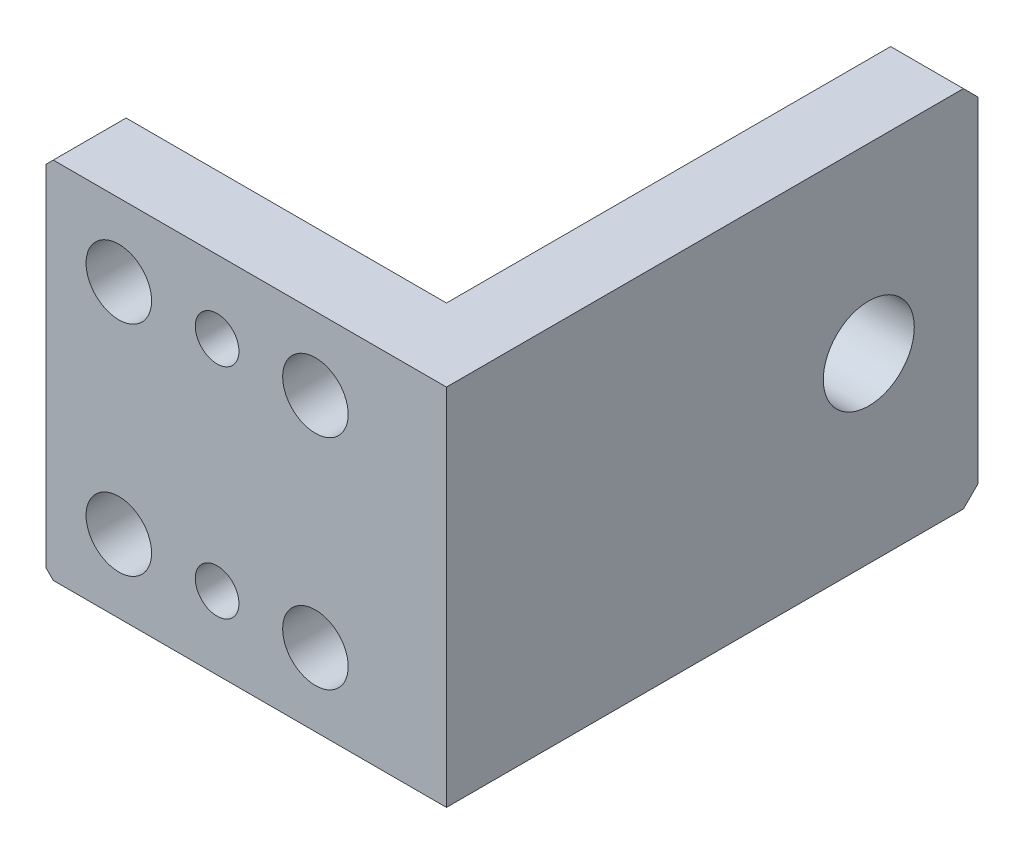
SolidWorks part; units mm, degrees
material "Q235-A"
ref_plane "Front Plane" through (0, 0, 0) normal (0, 0, 1) x (1, 0, 0)
ref_plane "Top Plane" through (0, 0, 0) normal (0, 1, 0) x (1, 0, 0)
ref_plane "Right Plane" through (0, 0, 0) normal (1, 0, 0) x (0, 0, -1)
sketch "Sketch1" plane through (0, 0, 0) normal (0, 0, 1) x (1, 0, 0)
  line L1 (-27.5, 25) -> (27.5, 25)
  line L2 (-27.5, 25) -> (-27.5, -25)
  line L3 (-27.5, -25) -> (27.5, -25)
  line L4 (27.5, 25) -> (27.5, -25)
  line L5 (-27.5, 25) -> (27.5, -25) construction
  line L6 (-27.5, -25) -> (27.5, 25) construction
  point P0 (0, 0)
  dimension "D1" = 55
  dimension "D2" = 50
extrude "Boss-Extrude1" add sketch "Sketch1" along normal blind 10
sketch "Sketch4" plane through (0, 0, 0) normal (0, 0, -1) x (-1, 0, 0)
  line L0 (-27.5, 25) -> (27.5, 25) construction
  line L1 (-17.5, 25) -> (-27.5, 25)
  line L2 (-17.5, 25) -> (-17.5, -25)
  line L3 (-17.5, -25) -> (-27.5, -25)
  line L4 (-27.5, 25) -> (-27.5, -25)
  line L5 (27.5, -25) -> (-27.5, -25) construction
  line L6 (-27.5, -25) -> (-27.5, 25) construction
  dimension "D1" = 10
extrude "Boss-Extrude2" add sketch "Sketch4" along normal blind 63
hole_wizard "M8 Clearance Hole1" positions "Sketch6" profile "Sketch7" hole size "M8" standard "GB"
sketch "Sketch6" plane through (0, 0, 0) normal (0, 0, -1) x (-1, 0, 0)
  line L0 (27.5, 0) -> (-40.8743, 0) construction
  line L1 (27.5, 25) -> (27.5, -25) construction
  line L3 (-17.5, -25) -> (-17.5, 25) construction
  point P0 (17.5, -15)
  point P2 (17.5, 15)
  point P4 (-9.5, -15)
  point P6 (-9.5, 15)
  dimension "D1" = 30
  dimension "D2" = 27
  dimension "D3" = 8
sketch "Sketch7" plane through (-17.5, -15, 0) normal (1, 0, 0) x (0, 1, 0)
  line L0 (0, 0) -> (0, 123.7039)
  line L1 (0, 123.7039) -> (4.5, 121)
  line L2 (4.5, 121) -> (4.5, 0)
  line L5 (4.5, 0) -> (0, 0)
  line L10 (0, 123.7039) -> (-4.5, 121) construction
  line L11 (0, -6.35) -> (0, 107.95) construction
  dimension "孔直径" = 9
  dimension "孔深度" = 121
  dimension "导头角度" = 118
chamfer "Chamfer1" distance 1 angle 45 2 edges at (-27.5, -25, 5) (-27.5, 25, 5)
hole_wizard "M14x1.5 Tapped Hole1" positions "Sketch9" profile "Sketch10" tap size "M14x1.5" standard "GB" end condition through all
sketch "Sketch9" plane through (27.5, 0, 0) normal (1, 0, 0) x (0, 0, -1)
  line L0 (-10, 0) -> (102.6904, 0)
  line L1 (-10, -25) -> (-10, 25) construction
  line L2 (63, 25) -> (63, -25) construction
  point P0 (48, 0)
  dimension "D1" = 15
sketch "Sketch10" plane through (27.5, 0, -48) normal (0, 1, 0) x (0, 0, -1)
  line L0 (0, 0) -> (0, 55)
  line L1 (0, 55) -> (6.25, 55)
  line L2 (6.25, 55) -> (6.25, 0)
  line L5 (6.25, 0) -> (0, 0)
  line L11 (0, -6.35) -> (0, 107.95) construction
  dimension "通孔螺纹孔钻头直径" = 12.5
  dimension "通孔螺纹孔钻头深度" = 55
cosmetic thread "Cosmetic thread 1" parameters "D2"=14
chamfer "Chamfer2" distance 2 angle 45 2 edges at (22.5, 25, -63) (22.5, -25, -63)
hole_wizard "Size mm blind dowel hole 1" positions "Sketch11" profile "Sketch12" hole size "Ø6.0" standard "GB" end condition through all
sketch "Sketch11" plane through (0, 0, 0) normal (0, 0, -1) x (-1, 0, 0)
  line L0 (-27.5, 0) -> (55.4, 0)
  line L1 (-27.5, 23) -> (-27.5, -23) construction
  line L4 (-9.5, 15) -> (17.5, 15)
  line L7 (-9.5, -15) -> (17.5, -15)
  line L10 (4, 15) -> (4, -15)
  point P0 (4, -15)
  point P2 (4, 15)
  dimension "D1" = 0
  dimension "D2" = 0
sketch "Sketch12" plane through (-4, -15, 0) normal (1, 0, 0) x (0, 1, 0)
  line L0 (0, 0) -> (0, 10)
  line L1 (0, 10) -> (3, 10)
  line L2 (3, 10) -> (3, 0)
  line L5 (3, 0) -> (0, 0)
  line L11 (0, -6.35) -> (0, 107.95) construction
  dimension "通孔孔直径" = 6
  dimension "通孔孔深度" = 10
